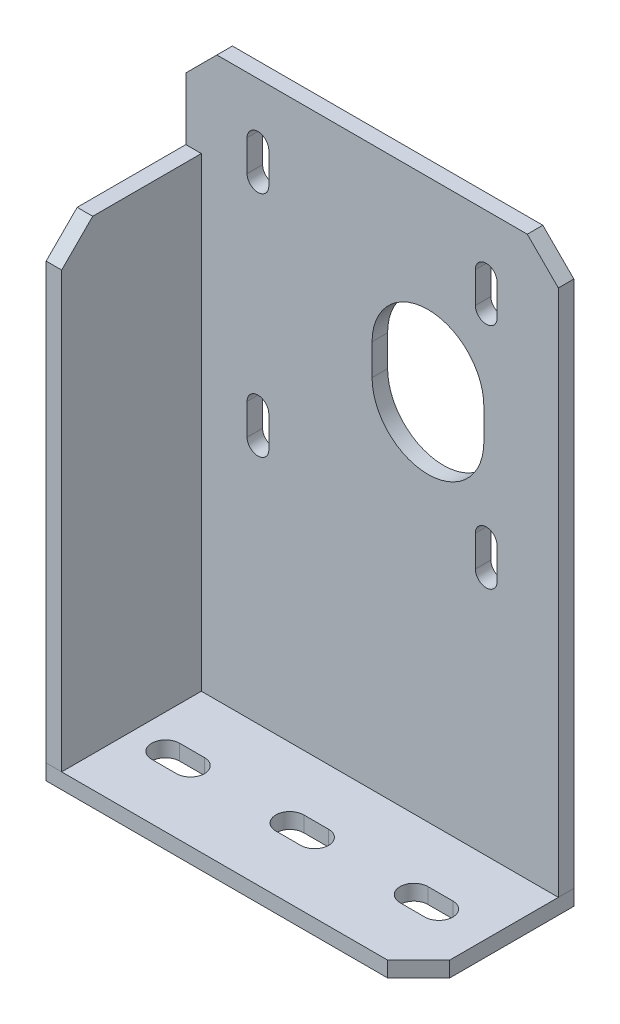
SolidWorks part; units mm, degrees
material "普通碳钢"
ref_plane "前视" through (0, 0, 0) normal (0, 0, 1) x (1, 0, 0)
ref_plane "上视" through (0, 0, 0) normal (0, 1, 0) x (1, 0, 0)
ref_plane "右视" through (0, 0, 0) normal (1, 0, 0) x (0, 0, -1)
sketch "草图1" plane through (0, 0, 0) normal (0, 1, 0) x (1, 0, 0)
  line L1 (-60, -25) -> (60, -25)
  line L2 (-60, -25) -> (-60, 25)
  line L3 (-60, 25) -> (60, 25)
  line L4 (60, -25) -> (60, 25)
  line L5 (-60, -25) -> (60, 25) construction
  line L6 (-60, 25) -> (60, -25) construction
  point P0 (0, 0)
  dimension "D1" = 120
  dimension "D2" = 50
extrude "凸台-拉伸1" add sketch "草图1" along normal blind 5
sketch "草图2" plane through (0, 5, 0) normal (0, 1, 0) x (1, 0, 0)
  line L0 (60, -25) -> (60, 25) construction
  line L1 (-60, 25) -> (60, 25)
  line L2 (-60, 25) -> (-60, 20)
  line L3 (-60, 20) -> (60, 20)
  line L4 (60, 25) -> (60, 20)
  dimension "D1" = 5
extrude "凸台-拉伸2" add sketch "草图2" along normal blind 180 separate body
sketch "草图3" plane through (0, 0, -20) normal (0, 0, 1) x (1, 0, 0)
  line L0 (0, 185) -> (0, 35.783) construction
  line L1 (-60, 185) -> (60, 185) construction
  line L2 (0, 125) -> (-36.7696, 161.7696) construction
  line L3 (0, 125) -> (36.7696, 161.7696) construction
  line L4 (36.7696, 161.7696) -> (-36.7696, 161.7696) construction
  line L5 (0, 125) -> (-52, 125) construction
  line L6 (-36.7696, 83.2304) -> (-36.7696, 93.2304) construction
  line L7 (-40.2696, 83.2304) -> (-40.2696, 93.2304)
  line L8 (-33.2696, 83.2304) -> (-33.2696, 93.2304)
  line L9 (36.7696, 83.2304) -> (36.7696, 93.2304) construction
  line L10 (33.2696, 83.2304) -> (33.2696, 93.2304)
  line L11 (40.2696, 83.2304) -> (40.2696, 93.2304)
  line L12 (36.7696, 156.7696) -> (36.7696, 166.7696) construction
  line L13 (33.2696, 156.7696) -> (33.2696, 166.7696)
  line L14 (40.2696, 156.7696) -> (40.2696, 166.7696)
  line L15 (-36.7696, 156.7696) -> (-36.7696, 166.7696) construction
  line L16 (-40.2696, 156.7696) -> (-40.2696, 166.7696)
  line L17 (-33.2696, 156.7696) -> (-33.2696, 166.7696)
  line L18 (18, 120) -> (18, 130) construction
  line L19 (0, 120) -> (0, 130)
  line L20 (36, 120) -> (36, 130)
  circle A0 centre (0, 125) radius 52 construction
  circle A1 centre (-36.7696, 161.7696) radius 3.5 construction
  circle A2 centre (36.7696, 161.7696) radius 3.5 construction
  circle A3 centre (36.7696, 88.2304) radius 3.5 construction
  circle A4 centre (-36.7696, 88.2304) radius 3.5 construction
  arc A5 (-40.2696, 83.2304) -> (-33.2696, 83.2304) centre (-36.7696, 83.2304) ccw
  arc A6 (-33.2696, 93.2304) -> (-40.2696, 93.2304) centre (-36.7696, 93.2304) ccw
  arc A7 (33.2696, 83.2304) -> (40.2696, 83.2304) centre (36.7696, 83.2304) ccw
  arc A8 (40.2696, 93.2304) -> (33.2696, 93.2304) centre (36.7696, 93.2304) ccw
  arc A9 (33.2696, 156.7696) -> (40.2696, 156.7696) centre (36.7696, 156.7696) ccw
  arc A10 (40.2696, 166.7696) -> (33.2696, 166.7696) centre (36.7696, 166.7696) ccw
  arc A11 (-40.2696, 156.7696) -> (-33.2696, 156.7696) centre (-36.7696, 156.7696) ccw
  arc A12 (-33.2696, 166.7696) -> (-40.2696, 166.7696) centre (-36.7696, 166.7696) ccw
  arc A13 (0, 120) -> (36, 120) centre (18, 120) ccw
  arc A14 (36, 130) -> (0, 130) centre (18, 130) ccw
  point P18 (-36.7696, 88.2304)
  point P24 (36.7696, 88.2304)
  point P31 (36.7696, 161.7696)
  point P38 (-36.7696, 161.7696)
  point P46 (18, 125)
  dimension "D1" = 104
  dimension "D4" = 7
  dimension "D5" = 7
  dimension "D6" = 3.5
  dimension "D7" = 3.5
  dimension "D8" = 3.5
  dimension "D9" = 3.5
  dimension "D15" = 18
  dimension "D2" = 60
  dimension "D3" = 90
  dimension "D10" = 10
  dimension "D11" = 10
  dimension "D12" = 10
  dimension "D13" = 10
  dimension "D14" = 18
  dimension "D16" = 10
extrude "切除-拉伸1" cut sketch "草图3" against normal blind 150
chamfer "倒角1" distance 10 angle 45 2 edges at (60, 185, -22.5) (-60, 185, -22.5)
sketch "草图4" plane through (0, 0, -20) normal (0, 0, 1) x (1, 0, 0)
  line L0 (36, 125) -> (0, 125)
  line L1 (36, 120) -> (36, 130) construction
  line L2 (0, 130) -> (0, 120) construction
  circle A0 centre (18, 125) radius 18
sketch "草图5" plane through (-60, 0, 0) normal (-1, 0, 0) x (0, 0, 1)
  line L0 (25, 5) -> (25, 0) construction
  line L1 (-20, 5) -> (25, 5)
  line L2 (-20, 5) -> (-20, 155)
  line L3 (-20, 155) -> (25, 155)
  line L4 (25, 5) -> (25, 155)
  dimension "D1" = 0
  dimension "D2" = 150
extrude "凸台-拉伸3" add sketch "草图5" against normal blind 5 separate body
chamfer "倒角2" distance 10 angle 45 1 edges at (-57.5, 155, 25)
sketch "草图6" plane through (0, 0, -25) normal (0, 0, -1) x (-1, 0, 0)
  line L0 (0, 185) -> (0, 20.4468) construction
  line L1 (-50, 185) -> (50, 185) construction
  line L3 (-40, 27.5) -> (40, 27.5)
  line L4 (-40, 27.5) -> (-40, 42.5)
  line L5 (-40, 42.5) -> (40, 42.5)
  line L6 (40, 27.5) -> (40, 42.5)
  line L7 (-40, 27.5) -> (40, 42.5) construction
  line L8 (-40, 42.5) -> (40, 27.5) construction
  point P5 (0, 35)
  dimension "D1" = 15
  dimension "D2" = 80
  dimension "D3" = 150
extrude "凸台-拉伸4" add sketch "草图6" along normal blind 20
sketch "草图9" plane through (0, 5, 0) normal (0, 1, 0) x (1, 0, 0)
  line L0 (-55, -2.5) -> (72.6808, -2.5) construction
  line L1 (-55, 20) -> (-55, -25) construction
  line L2 (-44, -2.5) -> (-36, -2.5) construction
  line L3 (-44, 2) -> (-36, 2)
  line L4 (-44, -7) -> (-36, -7)
  line L5 (-4, -2.5) -> (4, -2.5) construction
  line L6 (-4, 2) -> (4, 2)
  line L7 (-4, -7) -> (4, -7)
  line L8 (36, -2.5) -> (44, -2.5) construction
  line L9 (36, 2) -> (44, 2)
  line L10 (36, -7) -> (44, -7)
  line L11 (60, -25) -> (60, 25) construction
  arc A0 (-44, 2) -> (-44, -7) centre (-44, -2.5) ccw
  arc A1 (-36, -7) -> (-36, 2) centre (-36, -2.5) ccw
  arc A2 (-4, 2) -> (-4, -7) centre (-4, -2.5) ccw
  arc A3 (4, -7) -> (4, 2) centre (4, -2.5) ccw
  arc A4 (36, 2) -> (36, -7) centre (36, -2.5) ccw
  arc A5 (44, -7) -> (44, 2) centre (44, -2.5) ccw
  point P6 (-40, -2.5)
  point P12 (0, -2.5)
  point P19 (40, -2.5)
  dimension "D3" = 4.5
  dimension "D4" = 4.5
  dimension "D7" = 4.5
  dimension "D1" = 20
  dimension "D2" = 8
  dimension "D5" = 8
  dimension "D6" = 8
  dimension "D8" = 60
  dimension "D9" = 100
extrude "切除-拉伸2" cut sketch "草图9" against normal blind 20
chamfer "倒角3" distance 10 angle 45 1 edges at (60, 2.5, 25)
sketch "草图10" plane through (0, 27.5, 0) normal (0, -1, 0) x (1, 0, 0)
  line L0 (-40, -35) -> (40, -35) construction
  line L1 (-40, -45) -> (-40, -25) construction
  line L2 (40, -45) -> (40, -25) construction
  circle A0 centre (-25, -35) radius 4.5
  circle A1 centre (25, -35) radius 4.5
  dimension "D3" = 9
  dimension "D4" = 9
  dimension "D1" = 15
  dimension "D2" = 15
extrude "切除-拉伸3" cut sketch "草图10" against normal blind 20
